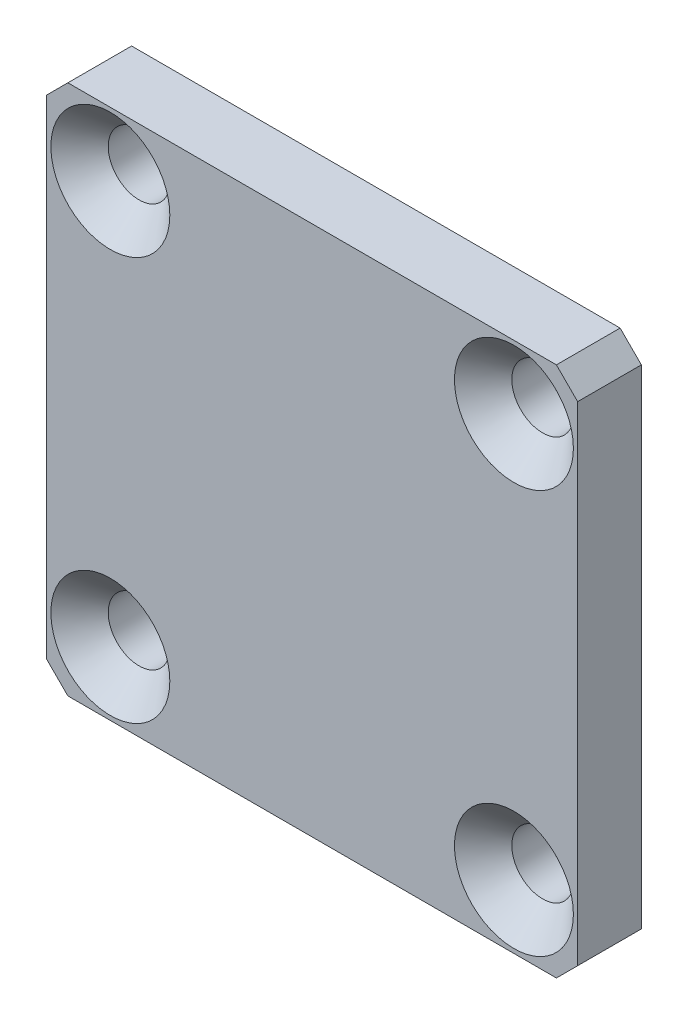
from build123d import *

# Parameters (mm, degrees)
SKETCH_1_W                   = 50
SKETCH_1_H                   = 50
EXTRUDE_1_DEPTH              = 3
HOLE_WIZARD_M5_1_D           = 5.8
HOLE_WIZARD_M5_1_CSINK_D     = 11.2
HOLE_WIZARD_M5_1_CSINK_ANGLE = 90
CHAMFER_1_SIZE               = 2
SKETCH_8_R                   = 19.2
SKETCH_8_R_2                 = 16.8
CUT_EXTRUDE_2_DEPTH          = 1.5


with BuildPart() as part:
    # 草图1 → 凸台-拉伸1 (new, symmetric)
    with BuildSketch(Plane.XY):
        Rectangle(SKETCH_1_W, SKETCH_1_H)
    extrude(amount=EXTRUDE_1_DEPTH, both=True)

    # M5 六角凹锥坑螺钉的锥形沉头孔1 (through all)
    with Locations(Plane.XY.offset(3)):
        with Locations((-19, 19), (19, 19), (-19, -19), (19, -19)):
            CounterSinkHole(HOLE_WIZARD_M5_1_D / 2, HOLE_WIZARD_M5_1_CSINK_D / 2, counter_sink_angle=HOLE_WIZARD_M5_1_CSINK_ANGLE)

    # 倒角1
    chamfer_1_edges = [part.edges().sort_by_distance(p)[0] for p in [
        (25, -25, 0),
        (-25, -25, 0),
        (-25, 25, 0),
        (25, 25, 0),
    ]]
    chamfer(chamfer_1_edges, length=CHAMFER_1_SIZE)

    # 草图8 → 切除-拉伸2 (cut)
    with BuildSketch(Plane(origin=(0, 0, -3), x_dir=(-1, 0, 0), z_dir=(0, 0, -1))):
        Circle(SKETCH_8_R)
        Circle(SKETCH_8_R_2, mode=Mode.SUBTRACT)
    extrude(amount=-CUT_EXTRUDE_2_DEPTH, mode=Mode.SUBTRACT)


solid = part.part
